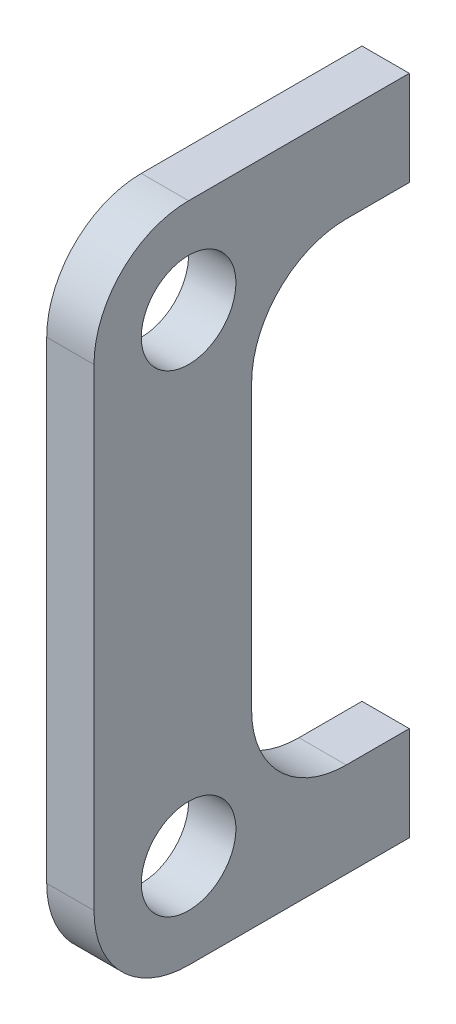
from build123d import *

# Parameters (mm, degrees)
BOSS_EXTRUDE1_DEPTH     = 15
CUT_EXTRUDE1_DEPTH      = 196.228071752
CUT_EXTRUDE1_DEPTH_BACK = 196.228071752
SKETCH3_R               = 15


with BuildPart() as part:
    # Sketch2 → Boss-Extrude1 (new body)
    with BuildSketch(Plane.ZY.offset(215.412167325)):
        with BuildLine():
            Line((0, -13), (20, -13))
            ThreePointArc((20, -13), (41.213203436, -4.213203436), (50, 17))
            Line((50, 17), (50, 107))
            ThreePointArc((50, 107), (41.213203436, 128.213203436), (20, 137))
            Line((20, 137), (0, 137))
            Line((0, 137), (0, 167))
            Line((0, 167), (70, 167))
            ThreePointArc((70, 167), (91.213203436, 158.213203436), (100, 137))
            Line((100, 137), (100, -13))
            ThreePointArc((100, -13), (91.213203436, -34.213203436), (70, -43))
            Line((70, -43), (0, -43))
            Line((0, -43), (0, -13))
        make_face()
    extrude(amount=BOSS_EXTRUDE1_DEPTH)

    # Sketch3 → Cut-Extrude1 (cut, two sides: drawn at the far end of the back side and taken through both)
    with BuildSketch(Plane.ZY.offset(230.412167325).offset(-CUT_EXTRUDE1_DEPTH_BACK)):
        with Locations((70, -13)):
            Circle(SKETCH3_R)
        with Locations((70, 137)):
            Circle(SKETCH3_R)
    extrude(amount=CUT_EXTRUDE1_DEPTH + CUT_EXTRUDE1_DEPTH_BACK, mode=Mode.SUBTRACT)


solid = part.part
